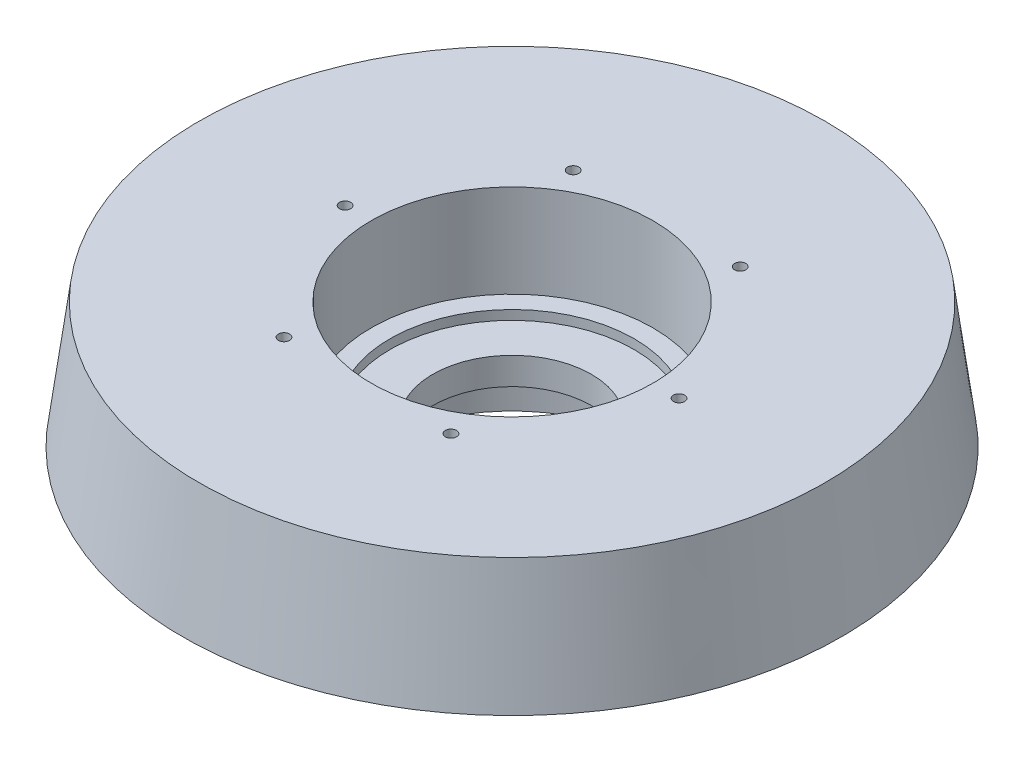
from build123d import *

# Parameters (mm, degrees)
CIRPATTERN1_COUNT = 6
CIRPATTERN2_COUNT = 6


with BuildPart() as part:
    # Sketch1 → Revolve1 (revolve)
    with BuildSketch(Plane.XY, mode=Mode.PRIVATE) as revolve1_sk:
        Polygon((-135, 0), (-135, 53), (-117, 53), (-117, 62), (-76, 62), (-76, 88), (-117, 88), (-117, 97), (-135, 97), (-135, 186), (-300, 186), (-315.79829971, 66), (-185, 66), (-185, 0), align=None)
    revolve(revolve1_sk.sketch.rotate(Axis((0, 0, 0), (0, 1, 0)), 270), axis=Axis((0, 0, 0), (0, 1, 0)))

    # Sketch3 → 1/2-13 Tapped Hole1 (revolve, cut)
    with BuildSketch(Plane(origin=(160, 186, 0), x_dir=(0, 0, 1), z_dir=(1, 0, 0))):
        Polygon((0, 0), (0, 28.619489309), (5.35813, 25.4), (5.35813, 0), align=None)
    f_1_2_13_tapped_hole1 = revolve(axis=Axis((160, 192.35, 0), (0, -1, 0)), mode=Mode.SUBTRACT)

    # CirPattern1: 1/2-13 Tapped Hole1 ×6 about axis
    cirpattern1_axis = Axis((0, 0, 0), (0, 1, 0))
    for i in range(1, CIRPATTERN1_COUNT):
        add(f_1_2_13_tapped_hole1.rotate(cirpattern1_axis, i * 360 / CIRPATTERN1_COUNT), mode=Mode.SUBTRACT)

    # Sketch5 → 1/2-13 Tapped Hole2 (revolve, cut)
    with BuildSketch(Plane(origin=(160, 0, 0), x_dir=(0, 0, -1), z_dir=(1, 0, 0))):
        Polygon((0, 0), (0, 34.479489309), (5.35813, 31.26), (5.35813, 0), align=None)
    f_1_2_13_tapped_hole2 = revolve(axis=Axis((160, -6.35, 0), (0, 1, 0)), mode=Mode.SUBTRACT)

    # CirPattern2: 1/2-13 Tapped Hole2 ×6 about axis
    cirpattern2_axis = Axis((0, 0, 0), (0, 1, 0))
    for i in range(1, CIRPATTERN2_COUNT):
        add(f_1_2_13_tapped_hole2.rotate(cirpattern2_axis, i * 360 / CIRPATTERN2_COUNT), mode=Mode.SUBTRACT)


solid = part.part
